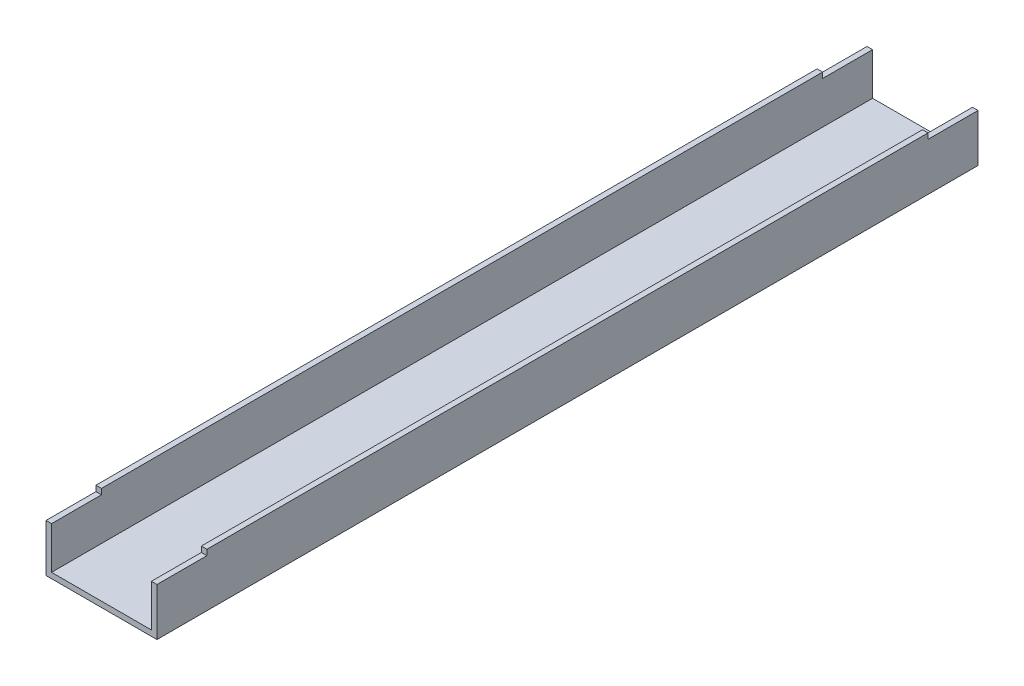
from build123d import *

# Parameters (mm, degrees)
EXTRUDE_1_DEPTH     = 740
SKETCH_2_W          = 100
SKETCH_2_H          = 5
CUT_EXTRUDE_1_DEPTH = 45
SKETCH_3_W          = 100
SKETCH_3_H          = 5
CUT_EXTRUDE_2_DEPTH = 45
CUT_EXTRUDE_3_DEPTH = 25
CUT_EXTRUDE_4_DEPTH = 25
SKETCH_8_W          = 5
SKETCH_8_H          = 5
CUT_EXTRUDE_5_DEPTH = 25
SKETCH_9_W          = 5
SKETCH_9_H          = 5
CUT_EXTRUDE_6_DEPTH = 25
EXTRUDE_2_DEPTH     = 25
SKETCH_11_W         = 5
SKETCH_11_H         = 5
EXTRUDE_3_DEPTH     = 25
EXTRUDE_4_DEPTH     = 25
SKETCH_13_W         = 5
SKETCH_13_H         = 5
EXTRUDE_5_DEPTH     = 25


with BuildPart() as part:
    # 草图1 → 凸台-拉伸1 (new body)
    with BuildSketch(Plane.XY):
        Polygon((0, 0), (100, 0), (100, 48), (95, 48), (95, 5), (5, 5), (5, 48), (0, 48), align=None)
    extrude(amount=EXTRUDE_1_DEPTH)

    # 草图2 → 切除-拉伸1 (cut)
    with BuildSketch(Plane(origin=(0, 0, 0), x_dir=(-1, 0, 0), z_dir=(0, 0, -1))):
        with Locations((-50, 45.5)):
            Rectangle(SKETCH_2_W, SKETCH_2_H)
    extrude(amount=-CUT_EXTRUDE_1_DEPTH, mode=Mode.SUBTRACT)

    # 草图3 → 切除-拉伸2 (cut)
    with BuildSketch(Plane.XY.offset(740)):
        with Locations((50, 45.5)):
            Rectangle(SKETCH_3_W, SKETCH_3_H)
    extrude(amount=-CUT_EXTRUDE_2_DEPTH, mode=Mode.SUBTRACT)

    # 草图6 → 切除-拉伸3 (cut)
    with BuildSketch(Plane(origin=(0, 0, 0), x_dir=(-1, 0, 0), z_dir=(0, 0, -1))):
        Polygon((-95, 43), (-100, 43), (-100, 0), (0, 0), (0, 43), (-5, 43), (-5, 5), (-95, 5), align=None)
    extrude(amount=-CUT_EXTRUDE_3_DEPTH, mode=Mode.SUBTRACT)

    # 草图7 → 切除-拉伸4 (cut)
    with BuildSketch(Plane.XY.offset(740)):
        Polygon((100, 0), (100, 43), (95, 43), (95, 5), (5, 5), (5, 43), (0, 43), (0, 0), align=None)
    extrude(amount=-CUT_EXTRUDE_4_DEPTH, mode=Mode.SUBTRACT)

    # 草图8 → 切除-拉伸5 (cut)
    with BuildSketch(Plane.XY.offset(695)):
        with Locations((97.5, 45.5)):
            Rectangle(SKETCH_8_W, SKETCH_8_H)
        with Locations((2.5, 45.5)):
            Rectangle(SKETCH_8_W, SKETCH_8_H)
    extrude(amount=-CUT_EXTRUDE_5_DEPTH, mode=Mode.SUBTRACT)

    # 草图9 → 切除-拉伸6 (cut)
    with BuildSketch(Plane(origin=(0, 0, 45), x_dir=(-1, 0, 0), z_dir=(0, 0, -1))):
        with Locations((-2.5, 45.5)):
            Rectangle(SKETCH_9_W, SKETCH_9_H)
        with Locations((-97.5, 45.5)):
            Rectangle(SKETCH_9_W, SKETCH_9_H)
    extrude(amount=-CUT_EXTRUDE_6_DEPTH, mode=Mode.SUBTRACT)

    # 草图10 → 凸台-拉伸2 (add)
    with BuildSketch(Plane(origin=(0, 0, 25), x_dir=(-1, 0, 0), z_dir=(0, 0, -1))):
        Polygon((-95, 5), (-95, 43), (-100, 43), (-100, 0), (0, 0), (0, 43), (-5, 43), (-5, 5), align=None)
    extrude(amount=EXTRUDE_2_DEPTH)

    # 草图11 → 凸台-拉伸3 (add)
    with BuildSketch(Plane(origin=(0, 0, 70), x_dir=(-1, 0, 0), z_dir=(0, 0, -1))):
        with Locations((-2.5, 45.5)):
            Rectangle(SKETCH_11_W, SKETCH_11_H)
        with Locations((-97.5, 45.5)):
            Rectangle(SKETCH_11_W, SKETCH_11_H)
    extrude(amount=EXTRUDE_3_DEPTH)

    # 草图12 → 凸台-拉伸4 (add)
    with BuildSketch(Plane.XY.offset(715)):
        Polygon((0, 0), (100, 0), (100, 43), (95, 43), (95, 5), (5, 5), (5, 43), (0, 43), align=None)
    extrude(amount=EXTRUDE_4_DEPTH)

    # 草图13 → 凸台-拉伸5 (add)
    with BuildSketch(Plane.XY.offset(670)):
        with Locations((2.5, 45.5)):
            Rectangle(SKETCH_13_W, SKETCH_13_H)
        with Locations((97.5, 45.5)):
            Rectangle(SKETCH_13_W, SKETCH_13_H)
    extrude(amount=EXTRUDE_5_DEPTH)


solid = part.part
